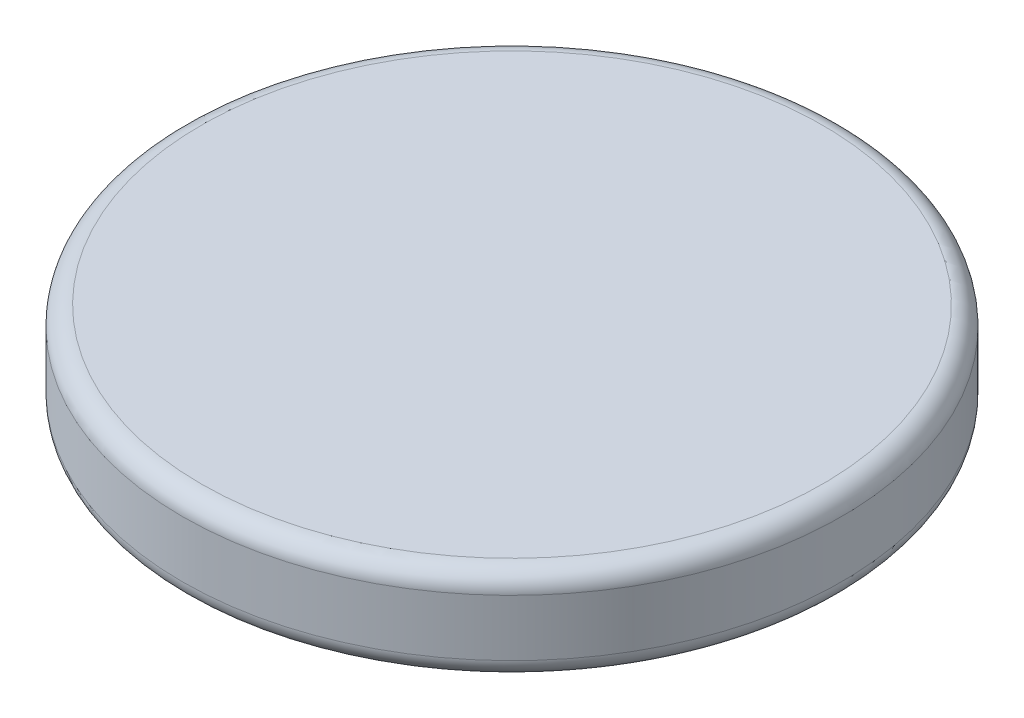
SolidWorks part; units mm, degrees
material "标准件"
ref_plane "前视基准面" through (0, 0, 0) normal (0, 0, 1) x (1, 0, 0)
ref_plane "上视基准面" through (0, 0, 0) normal (0, 1, 0) x (1, 0, 0)
ref_plane "右视基准面" through (0, 0, 0) normal (1, 0, 0) x (0, 0, -1)
sketch "草图1" plane through (0, 0, 0) normal (0, 1, 0) x (1, 0, 0)
  circle A0 centre (0, 0) radius 17.5
  dimension "D1" = 35
extrude "凸台-拉伸1" add sketch "草图1" along normal mid plane 5
fillet "圆角1" radius 1 2 edges at (0, -2.5, 17.5) (0, 2.5, 17.5)
